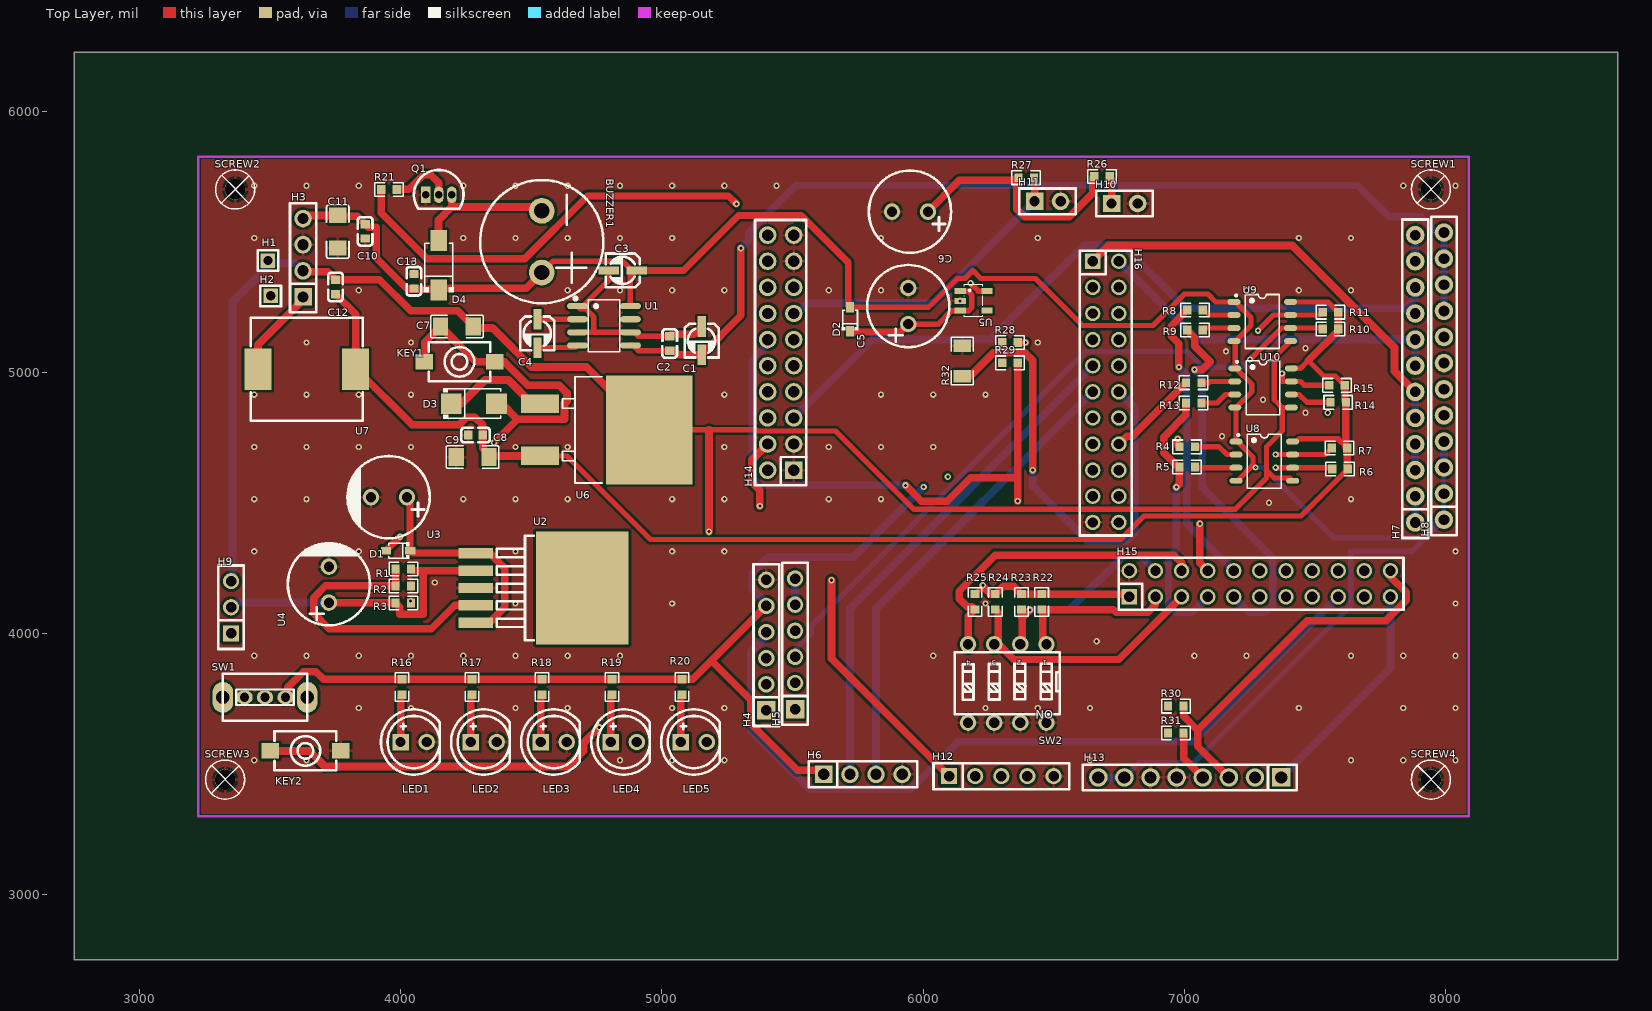
[diagram p0: Top Layer view]
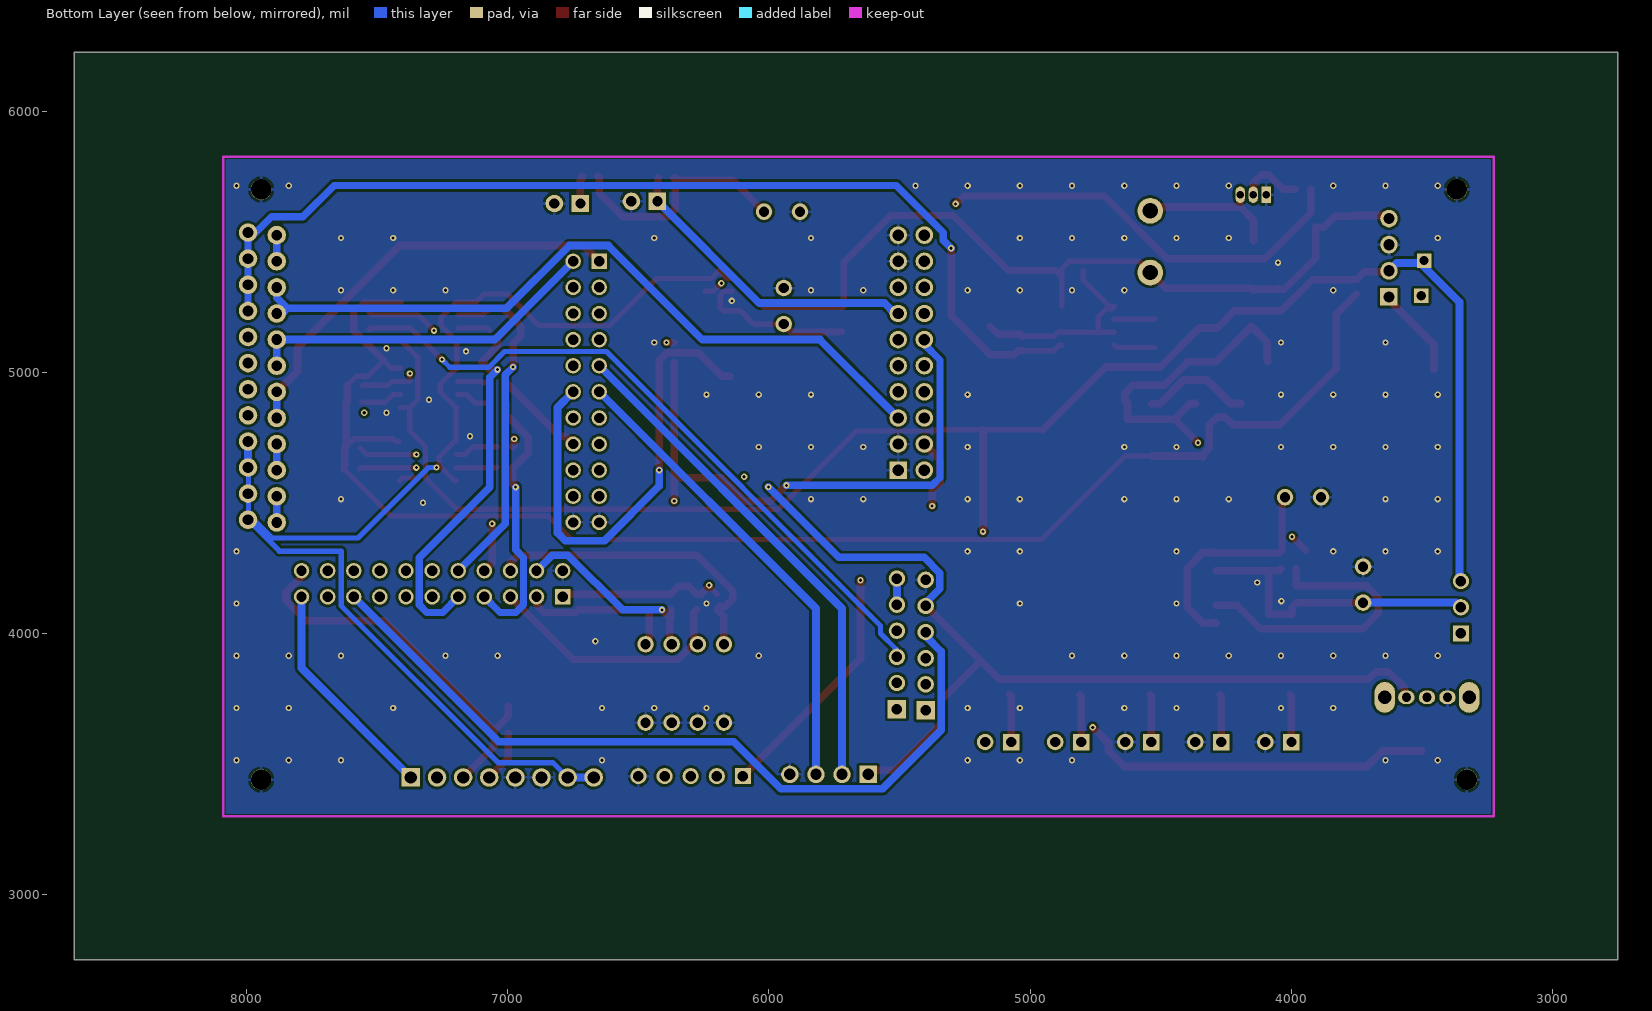
[diagram p1: Bottom Layer view, seen from below]
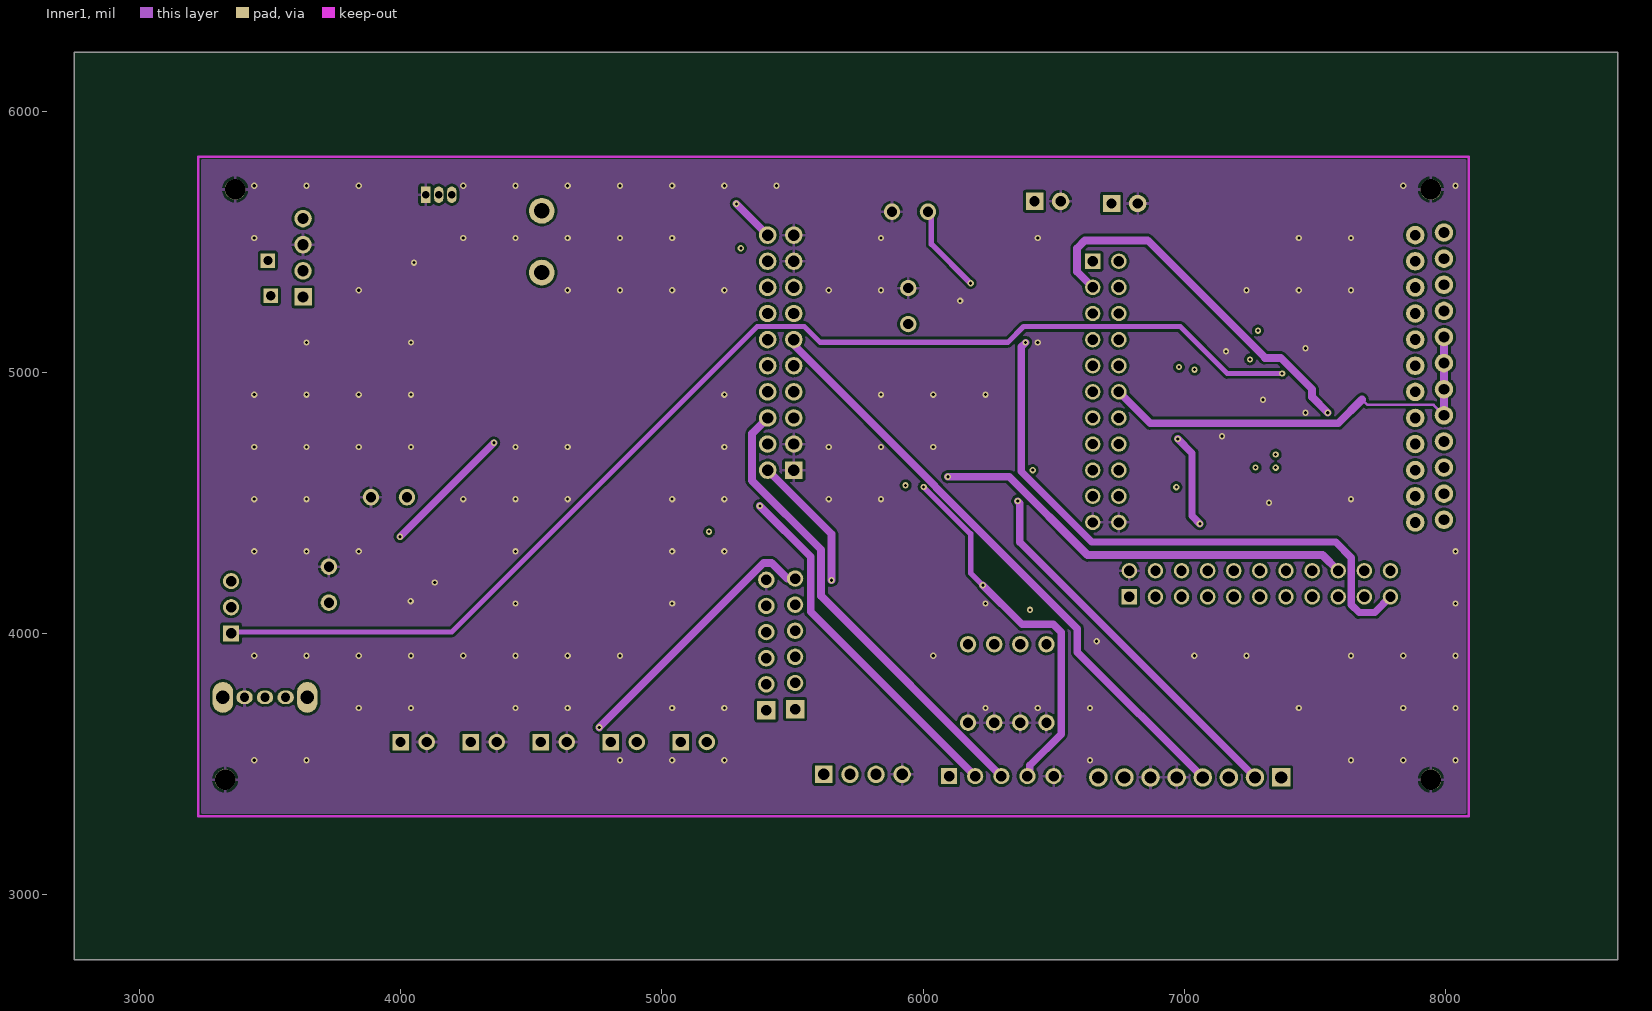
[diagram p2: Inner1]
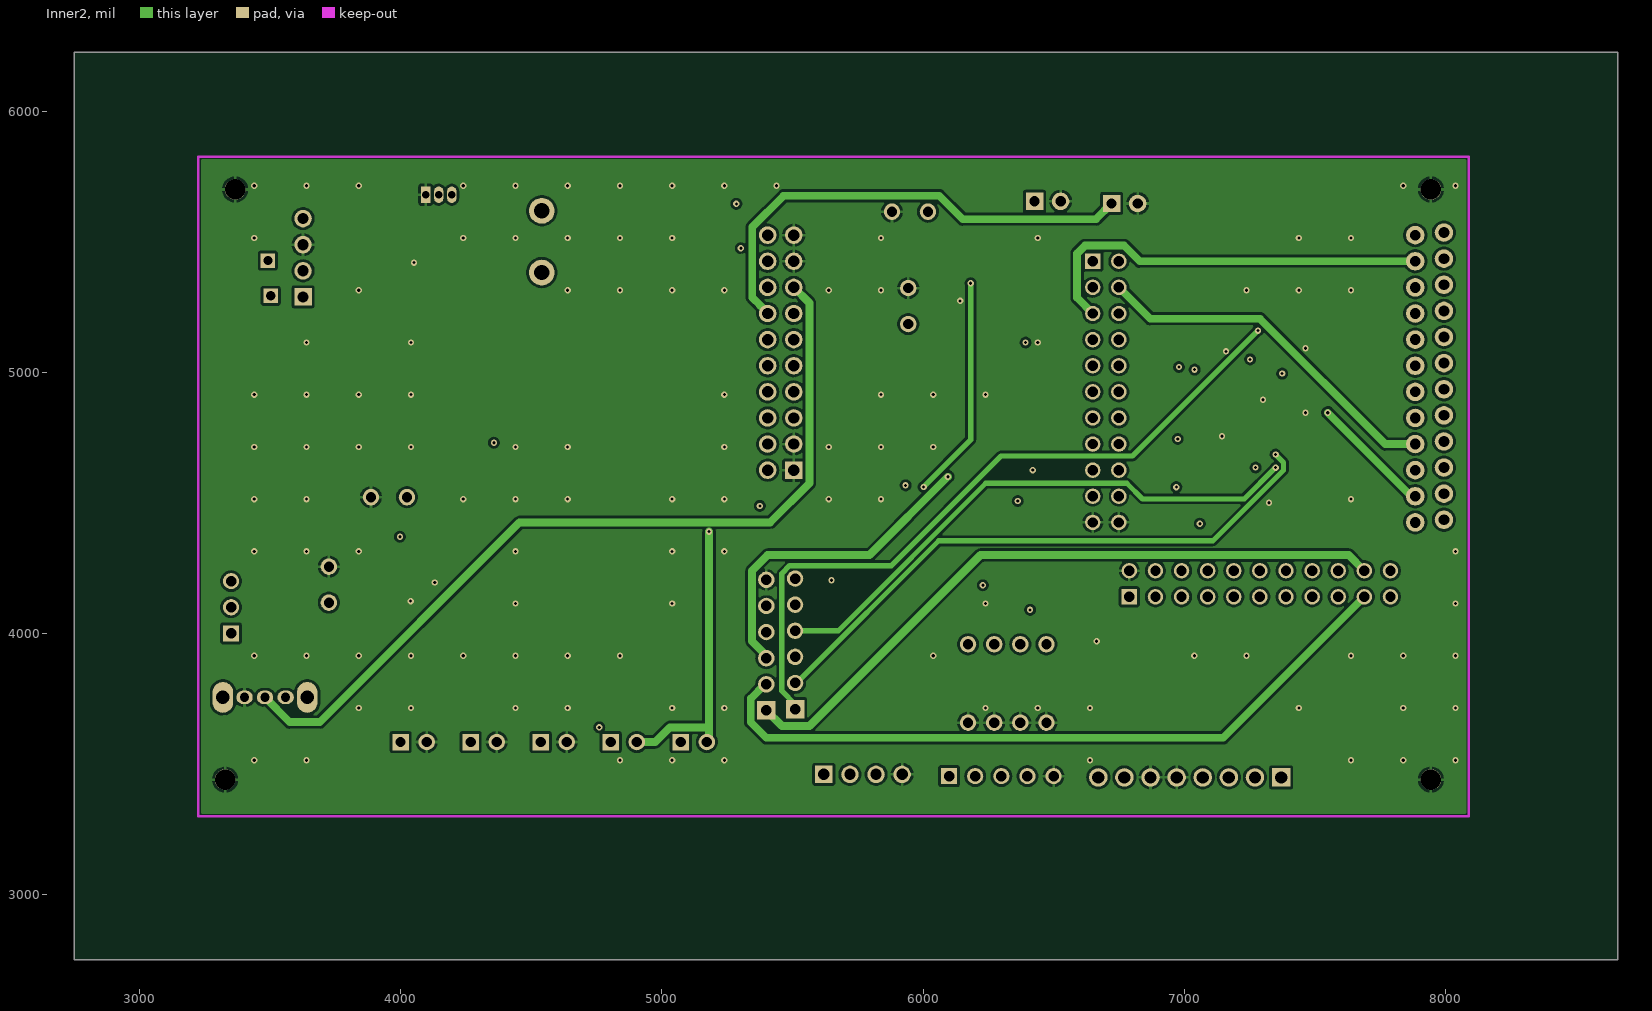
[diagram p3: Inner2]
# Altium PCB MISC75407.pcbdoc
Units mil, origin at the board's own origin, x right, y up, seen from the top; angles counter-clockwise.
Board outline 5910 x 3475 mil, 4 copper layers (Top Layer, Inner1, Inner2, Bottom Layer), stack 62.447 mil thick; 90 components, 74 nets, 316 pads, 149 vias.

## Layer stack, top to bottom
Top Layer: signal copper 1.378
Dielectric1: surface 8.283, 7628 RC49% 8.6mil, Dk 0
Inner1: signal copper 0.598
Dielectric2: surface 41.929, 1.1mm H/HOZ Copper, Dk 0
Inner2: signal copper 0.598
Dielectric3: surface 8.283, 7628 RC49% 8.6mil, Dk 0
Bottom Layer: signal copper 1.378

## Board outline
8660,2750 2750,2750 2750,6225 8660,6225

## Design rules (kind name [scope] priority, off if disabled: settings)
BoardOutlineClearance copperThickness2oz_1 [All] p2 off: genericclearance=7.99 ignorepadtopadclearanceinfootprint=FALSE except(0: Arc-SplitContinuation Track-SplitContinuation SMDPad-SplitContinuation THPad-SplitContinuation Via-SplitContinuation Fill-SplitContinuation Region-SplitContinuation Poly-SplitContinuation Text-SplitContinuation Hole-SplitContinuation; 5.98: Arc-CutoutEdge SMDPad-CutoutEdge THPad-CutoutEdge Via-CutoutEdge Fill-CutoutEdge Region-CutoutEdge Text-CutoutEdge; 6.93: Hole-OutlineEdge Hole-CutoutEdge; 10: Poly-OutlineEdge Poly-CutoutEdge; 11.81: Arc-OutlineEdge Track-OutlineEdge SMDPad-OutlineEdge THPad-OutlineEdge Via-OutlineEdge Fill-OutlineEdge Region-OutlineEdge Text-OutlineEdge Track-CutoutEdge)
BoardOutlineClearance copperThickness1oz_1 [All] p4: genericclearance=4.02 ignorepadtopadclearanceinfootprint=FALSE except(0: Arc-SplitContinuation Track-SplitContinuation SMDPad-SplitContinuation THPad-SplitContinuation Via-SplitContinuation Fill-SplitContinuation Region-SplitContinuation Poly-SplitContinuation Text-SplitContinuation Hole-SplitContinuation; 6: SMDPad-CutoutEdge THPad-CutoutEdge Via-CutoutEdge Fill-CutoutEdge Region-CutoutEdge Text-CutoutEdge; 6.93: Hole-OutlineEdge Hole-CutoutEdge; 10: Poly-OutlineEdge Poly-CutoutEdge; 11.8: Arc-OutlineEdge Track-OutlineEdge SMDPad-OutlineEdge THPad-OutlineEdge Via-OutlineEdge Fill-OutlineEdge Region-OutlineEdge Text-OutlineEdge; 11.81: Arc-CutoutEdge Track-CutoutEdge)
Clearance copperThickness2oz [All] p1 off: gap=7.99 ignorepadtopadclearanceinfootprint=FALSE except(5.98: SMDPad-Track SMDPad-SMDPad THPad-Track SMDPad-THPad THPad-THPad Track-Via SMDPad-Via THPad-Via Via-Via Fill-Track Region-Track Fill-SMDPad Region-SMDPad Fill-THPad Region-THPad Fill-Via Region-Via Fill-Fill Fill-Region Region-Region Arc-Track Arc-SMDPad Arc-THPad Arc-Via Fill-Arc Region-Arc Arc-Arc Text-Track SMDPad-Text Text-THPad Text-Via Fill-Text Region-Text Arc-Text Text-Text; 6.93: Hole-Track Hole-SMDPad Hole-THPad Hole-Via Fill-Hole Region-Hole Hole-Arc Hole-Text; 10: Poly-Track Poly-SMDPad Poly-THPad Poly-Via Poly-Fill Poly-Region Poly-Poly Poly-Arc Poly-Text Poly-Hole)
Clearance copperThickness1oz [All] p3: gap=4.02 ignorepadtopadclearanceinfootprint=FALSE except(5.98: SMDPad-Track SMDPad-SMDPad THPad-Track SMDPad-THPad THPad-THPad Track-Via SMDPad-Via THPad-Via Via-Via Fill-Track Region-Track Fill-SMDPad Region-SMDPad Fill-THPad Region-THPad Fill-Via Region-Via Fill-Fill Fill-Region Region-Region; 6: Arc-Track Arc-SMDPad Arc-THPad Arc-Via Fill-Arc Region-Arc Arc-Arc Text-Track SMDPad-Text Text-THPad Text-Via Fill-Text Region-Text Arc-Text Text-Text; 6.93: Hole-Track Hole-SMDPad Hole-THPad Hole-Via Fill-Hole Region-Hole Hole-Arc Hole-Text; 10: Poly-Track Poly-SMDPad Poly-THPad Poly-Via Poly-Fill Poly-Region Poly-Poly Poly-Arc Poly-Text Poly-Hole)
DiffPairsRouting differentialPair [All] p1: maxlimit=6 minlimit=6 mostfreqgap=6 toplayer_minwidth=5 toplayer_prefwidth=10 toplayer_maxwidth=100 toplayer_mingap=6 toplayer_prefgap=6 toplayer_maxgap=6 midlayer1_minwidth=5 midlayer1_prefwidth=10 midlayer1_maxwidth=100 midlayer1_mingap=6 midlayer1_prefgap=6 midlayer1_maxgap=6 midlayer2_minwidth=5 midlayer2_prefwidth=10 midlayer2_maxwidth=100 midlayer2_mingap=6 midlayer2_prefgap=6 midlayer2_maxgap=6 bottomlayer_minwidth=5 bottomlayer_prefwidth=10 bottomlayer_maxwidth=100 bottomlayer_mingap=6 bottomlayer_prefgap=6 bottomlayer_maxgap=6 maxuncoupledlength=10
HoleToHoleClearance otherClearance [All] p1: gap=11.81 allowstackedmicrovias=TRUE
Length netLength [All] p1: minlimit=0 maxlimit=0
MatchedLengths netLengthTolerance [All] p1: tolerance=1000
PasteMaskExpansion pasteMaskExpansion [All] p1: expansion=0
PlaneConnect innerPlane [All] p1: planeconnectstyle=Relief reliefexpansion=20 reliefentries=4 reliefconductorwidth=10 reliefairgap=10
PolygonConnect copperRegion [(InNet('GND'))] p1: connectstyle=Relief reliefconductorwidth=10 reliefentries=4 polygonreliefangle="90 Angle" airgapwidth=10 via.connectstyle=Relief via.reliefconductorwidth=10 via.reliefentries=4 via.polygonreliefangle="90 Angle" via.airgapwidth=10
RoutingVias viaSize [All] p1: holewidth=12.01 width=24.02 viastyle="Through Hole" minholewidth=11.81 minwidth=19.68 maxholewidth=248.03 maxwidth=393.7
SolderMaskExpansion solderMaskExpansion [IsVia] p1: expansion=-1000 istentingtop=TRUE
SolderMaskExpansion solderMaskExpansion [All] p2: expansion=2 istentingtop=FALSE
Width copperThickness2oz_2 [All] p1 off: maxlimit=100 minlimit=8 preferedwidth=10
Width copperThickness1oz_2 [All] p2: maxlimit=10 minlimit=10 preferedwidth=10 toplayer_minwidth=5 toplayer_maxwidth=100 toplayer_prefwidth=30 midlayer1_minwidth=5 midlayer1_maxwidth=100 midlayer1_prefwidth=30 midlayer2_minwidth=5 midlayer2_maxwidth=100 midlayer2_prefwidth=30 bottomlayer_minwidth=5 bottomlayer_maxwidth=100 bottomlayer_prefwidth=30

## Components (designator, comment, footprint, x,y, rotation, side; value= is the part's Value field where it differs from the comment)
BUZZER1 "buzzer" BUZ-TH_BD12.0-P6.00-D0.9-RD 4540,5500 r270 top
C1 "100uF" C_Ele_SMD_3x5.4mm 5151.69,5121.18 r90 top
C2 "100nF" C0603 5030,5110 r270 top
C3 "10uF" C_Ele_SMD_3x5.4mm 4849.45,5390.15 r0 top
C4 "47uF" C_Ele_SMD_3x5.4mm 4522.78,5148.38 r90 top
C5 "4.7uF" CAP-TH_BD8.0-P3.50-D0.5-FD_4.7UF400V8X14FS 5943.42,5253.46 r90 top
C6 "4.7uF" CAP-TH_BD8.0-P3.50-D0.5-FD_4.7UF400V8X14FS 5950,5615 r180 top
C7 "47UF" C1206 4215,5175 r0 top
C8 "100nF" C0603 4286.22,4759.27 r0 top
C9 "22UF" C1206 4275,4675 r0 top
C10 "100nF" C0603 3863.58,5539.45 r90 top
C11 "22UF" C1206 3758.58,5538.19 r90 top
C12 "4.7UF" C0603 3749.89,5326.65 r270 top
C13 "100nF" C0603 4050.19,5348.55 r270 top
D1 "1N5819WS" SOD-323_L1.8-W1.3-LS2.5-RD 3989.75,4316.72 r180 top
D2 "1N5819WS" SOD-323_L1.8-W1.3-LS2.5-RD 5720.39,5202.68 r90 top
D3 "SS34" SMA_L4.3-W2.6-LS5.2-RD 4280,4880 r0 top
D4 "SS34" SMA_L4.3-W2.6-LS5.0-RD 4145.32,5409.77 r90 top
H1 "" HDR-TH_1P-V-M_XKB_X4611WV-01I-C28D40 3491.11,5427.5 r90 top
H2 "" HDR-TH_1P-V-M_XKB_X4611WV-01I-C28D40 3501.86,5292.5 r90 top
H3 "" HDR-TH_4P-P2.54-V-F 3625.64,5438.48 r90 top
H4 "" HDR-TH_6P-P2.54-V-F 5400,3955 r90 top
H5 "" HDR-TH_6P-P2.54-V-F 5510,3960 r90 top
H6 "" HDR-TH_4P-P2.54-V-F 5770,3460 r0 top
H7 "" HDR-TH_12P-P2.54-V-F 7885,4975 r90 top
H8 "" HDR-TH_12P-P2.54-V-F 7995,4985 r90 top
H9 "" HDR-TH_3P-P2.54-V-F 3350,4100 r90 top
H10 "" HDR-TH_2P-P2.54-V-F 6771.95,5646.21 r0 top
H11 "" HDR-TH_2P-P2.54-V-F 6476.95,5654.61 r0 top
H12 "" HDR-TH_5P-P2.54-V-F 6299.85,3453.3 r0 top
H13 "" HDR-TH_8P-P2.54-V-F-1 7021.22,3448.3 r180 top
H14 "" HDR-TH_20P-P2.54-V-R2-C10-S2.54 5455,5075 r90 top
H15 "CS-1106-2*11B" HDR-TH_22P-P2.54-V-M-R2-C11-S2.54-1 7290,4190 r0 top
H16 "CS-1106-2*11B" HDR-TH_22P-P2.54-V-M-R2-C11-S2.54-1 6700,4925 r270 top
KEY1 "SW-SPST" KEY-SMD_L6.0-W3.6-LS8.0 4225,5040 r0 top
KEY2 "SW-SPST" KEY-SMD_L6.0-W3.6-LS8.0 3635,3550 r0 top
LED1 "" LED-TH_5mm 4049.26,3583.93 r0 top
LED2 "" LED-TH_5mm 4317.5,3583.93 r0 top
LED3 "" LED-TH_5mm 4585.73,3583.93 r0 top
LED4 "" LED-TH_5mm 4853.97,3583.93 r0 top
LED5 "" LED-TH_5mm 5122.21,3583.93 r0 top
Q1 "" S8050_TO_92 4145.32,5679.77 r0 top
R1 "3.9K" R0603 4009.75,4246.72 r0 top
R2 "1K" R0603 4009.75,4181.72 r180 top
R3 "1K" R0603 4009.75,4116.72 r180 top
R4 "1K" R0603 7011.46,4714.67 r180 top
R5 "1K" R0603 7011.46,4636.97 r180 top
R6 "1K" R0603 7597.22,4629.26 r0 top
R7 "1K" R0603 7595,4710 r0 top
R8 "1K" R0603 7041.46,5238.93 r180 top
R9 "1K" R0603 7041.46,5161.22 r180 top
R10 "1K" R0603 7560,5165 r0 top
R11 "1K" R0603 7560,5230 r0 top
R12 "1K" R0603 7036.46,4959.87 r180 top
R13 "1K" R0603 7036.46,4882.17 r180 top
R14 "1K" R0603 7590,4885 r0 top
R15 "1K" R0603 7585,4950 r0 top
R16 "1K" R0603 4004.26,3794.27 r90 top
R17 "1K" R0603 4272.5,3794.27 r90 top
R18 "1K" R0603 4540.73,3794.27 r90 top
R19 "3.3K" R0603 4808.97,3794.27 r90 top
R20 "3.3K" R0603 5077.21,3794.27 r90 top
R21 "1K" R0603 3955,5700 r0 top
R22 "1K" R0603 6454.43,4120.95 r270 top
R23 "1K" R0603 6376.73,4120.95 r270 top
R24 "1K" R0603 6276.73,4120.95 r270 top
R25 "1K" R0603 6199.03,4120.95 r270 top
R26 "1K" R0603 6685,5750 r0 top
R27 "1K" R0603 6395,5745 r0 top
R28 "1K" R0603 6333.02,5113.91 r0 top
R29 "1K" R0603 6333.02,5036.21 r0 top
R30 "1K" R0603 6968.02,3721.21 r0 top
R31 "1K" R0603 6968.02,3618.3 r0 top
R32 "100mΩ" R1206 6150.34,5042.73 r90 top
SCREW1 "" M2螺丝 7945,5700 r0 top
SCREW2 "" M2螺丝 3365.64,5700 r0 top
SCREW3 "" M2螺丝 3327.21,3440 r0 top
SCREW4 "" M2螺丝 7945,3440 r0 top
SW1 "" 拨动开关 3475,3755 r0 top
SW2 "DIP switch EI-04" SW-TH_DIPSWITCHEI-04 6322.49,3808.25 r180 top
U1 "LM2663M" SOIC-8_L4.9-W3.9-P1.27-LS6.0-BL 4778.16,5178.03 r270 top
U2 "MIC29302" TO-263-5_L10.1-W8.7-P1.70-LS15.2-BR 4491.27,4173.77 r180 top
U3 "22UF400V" CAP-TH_BD8.0-P3.50-D0.6-FD 3954.75,4521.72 r180 top
U4 "22UF400V" CAP-TH_BD8.0-P3.50-D0.6-FD 3724.75,4186.72 r90 top
U5 "TPS73633DBVR" SOT-23-5_L3.0-W1.7-P0.95-LS2.8-BR 6193.42,5273.46 r180 top
U6 "LM2940HR-5.0" TO-263-2_L10.1-W9.1-P5.08-LS15.2-BR 4742.21,4779.67 r180 top
U7 "6.8UH" IND-SMD_L10.9-W10.0_ACL1009 3639.89,5011.65 r180 top
U8 "HCPL-0631-000E" SO-8_L5.1-W3.9-P1.27-LS6.0-BL 7307.06,4659.67 r270 top
U9 "HCPL-0631-000E" SO-8_L5.1-W3.9-P1.27-LS6.0-BL 7299.26,5194.26 r270 top
U10 "HCPL-0631-000E" SO-8_L5.1-W3.9-P1.27-LS6.0-BL 7302.06,4939.87 r270 top

## Footprints (in the part's own frame and the unit in brackets; to place one, negate y for a bottom-side part, rotate by r counter-clockwise, add the part's x,y. Pads: shape width x height; smd on the part's side, far side on the other; paste and mask are expansions set on the pad)
BUZ-TH_BD12.0-P6.00-D0.9-RD [mm]
  round 2.5 hole 1.5 paste+0 mask+0.05: 1(-3,0) 2(3,0)
  silkscreen extent -5.99,-5.99 5.99,5.99
C0603 [mm]
  rect 0.8x0.9 smd: 1(-0.7,0) 2(0.7,0)
  silkscreen extent -1.39,-0.71 1.39,0.71
C1206 [mm]
  rect 1.485x1.728 smd paste-100 mask+0.051: 1(-1.593,0) 2(1.593,0)
  silkscreen extent -2.56,-1.09 2.56,1.09
C_Ele_SMD_3x5.4mm [mil]
  rect 78.7x31.5 smd paste+0 mask+2: 1(54.1,-0.55) 2(-53.7,-0.55)
  silkscreen extent -65,-65 65,65
CAP-TH_BD8.0-P3.50-D0.5-FD_4.7UF400V8X14FS [mm]
  round 1.6 hole 1: 1(-1.75,0) 2(1.75,0)
  silkscreen extent -4,-4 4,4
CAP-TH_BD8.0-P3.50-D0.6-FD [mm]
  round 1.6 hole 1: 1(-1.75,0) 2(1.75,0)
  silkscreen extent -3.96,-4 4.04,4
HDR-TH_1P-V-M_XKB_X4611WV-01I-C28D40 [mm]
  rect 1.4x1.4 hole 0.9: 1(0,0)
  silkscreen extent -1,-1 1,1
HDR-TH_2P-P2.54-V-F [mm]
  rect 1.7x1.7 hole 1: 1(-1.27,0)
  round 1.7 hole 1: 2(1.27,0)
  silkscreen extent -2.74,-1.25 2.74,1.25
HDR-TH_3P-P2.54-V-F [mil]
  rect 62x62 hole 40.16: 1(-100,0)
  round 62 hole 40.16: 2(0,0) 3(100,0)
  silkscreen extent -160,-49 160,49
HDR-TH_4P-P2.54-V-F [mm]
  rect 1.7x1.7 hole 1.1: 1(-3.81,0)
  round 1.7 hole 1.1: 2(-1.27,0) 3(1.27,0) 4(3.81,0)
  silkscreen extent -5.29,-1.27 5.29,1.27
HDR-TH_5P-P2.54-V-F [mil]
  rect 62x62 hole 40.16: 1(-200,0)
  round 62 hole 40.16: 2(-100,0) 3(0,0) 4(100,0) 5(200,0)
  silkscreen extent -260,-50 260,50
HDR-TH_6P-P2.54-V-F [mm]
  rect 1.8x1.8 hole 1.02: 1(-6.35,0)
  round 1.6 hole 1.02: 2(-3.81,0) 3(-1.27,0) 4(1.27,0) 5(3.81,0) 6(6.35,0)
  silkscreen extent -7.87,-1.25 7.87,1.25
HDR-TH_8P-P2.54-V-F-1 [mm]
  rect 1.8x1.8 hole 1.2: 1(-8.89,0)
  round 1.8 hole 1.2: 2(-6.35,0) 3(-3.81,0) 4(-1.27,0) 5(1.27,0) 6(3.81,0) 7(6.35,0) 8(8.89,0)
  silkscreen extent -10.41,-1.25 10.41,1.25
HDR-TH_12P-P2.54-V-F [mm]
  round 1.8 hole 1.05: 1(-13.97,0) 2(-11.43,0) 3(-8.89,0) 4(-6.35,0) 5(-3.81,0) 6(-1.27,0) 7(1.27,0) 8(3.81,0) 9(6.35,0) 10(8.89,0) 11(11.43,0) 12(13.97,0)
  silkscreen extent -15.49,-1.25 15.49,1.25
HDR-TH_20P-P2.54-V-R2-C10-S2.54 [mm]
  rect 1.7x1.7 hole 1.1: 1(-11.43,-1.27)
  round 1.7 hole 1.1: 2(-11.43,1.27) 3(-8.89,-1.27) 4(-8.89,1.27) 5(-6.35,-1.27) 6(-6.35,1.27) 7(-3.81,-1.27) 8(-3.81,1.27) 9(-1.27,-1.27) 10(-1.27,1.27) 11(1.27,-1.27) 12(1.27,1.27) 13(3.81,-1.27) 14(3.81,1.27) 15(6.35,-1.27) 16(6.35,1.27) 17(8.89,-1.27) 18(8.89,1.27) 19(11.43,-1.27) 20(11.43,1.27)
  silkscreen extent -12.9,-2.54 12.9,2.5
HDR-TH_22P-P2.54-V-M-R2-C11-S2.54-1 [mm]
  rect 1.5x1.5 hole 1: 1(-12.7,-1.27)
  round 1.5 hole 1: 2(-12.7,1.27) 3(-10.16,-1.27) 4(-10.16,1.27) 5(-7.62,-1.27) 6(-7.62,1.27) 7(-5.08,-1.27) 8(-5.08,1.27) 9(-2.54,-1.27) 10(-2.54,1.27) 11(0,-1.27) 12(0,1.27) 13(2.54,-1.27) 14(2.54,1.27) 15(5.08,-1.27) 16(5.08,1.27) 17(7.62,-1.27) 18(7.62,1.27) 19(10.16,-1.27) 20(10.16,1.27) 21(12.7,-1.27) 22(12.7,1.27)
  silkscreen extent -13.72,-2.54 13.97,2.54
IND-SMD_L10.9-W10.0_ACL1009 [mm]
  rect 2.6x4 smd: 1(-4.75,0) 2(4.75,0)
  silkscreen extent -5.45,-5 5.45,5
KEY-SMD_L6.0-W3.6-LS8.0 [mm]
  rect 1.7x1.5 smd: 1(-3.431,0) 2(3.431,0)
  silkscreen extent -3.01,-1.9 2.99,1.9
LED-TH_5mm [mm]
  rect 1.6x1.6 hole 1 paste+0 mask+0.051: 1(-1.27,0)
  round 1.6 hole 1 paste+0 mask+0.051: 2(1.27,0)
  silkscreen extent -3.17,-3.17 2.54,3.17
M2螺丝 [mm]
  round 2 hole 2: 1(0,0)
  silkscreen extent -1.9,-1.9 1.9,1.9
R0603 [mil]
  rect 31.75x34.02 smd paste-3937.01 mask+2: 1(-29.66,0) 2(29.66,0)
  silkscreen extent -55,-26 55,26
R1206 [mil]
  rect 47.54x66.97 smd paste-3937.01 mask+2: 1(-58.22,0) 2(58.22,0)
  silkscreen extent -91,-42 91,42
S8050_TO_92 [mil]
  rect 35.4x63 hole 27.6 paste+0 mask+2: 1(-50,0)
  oval 35.4x63 hole 27.6 paste+0 mask+2: 2(0,0) 3(50,0)
  silkscreen extent -95,-53 95,95
SMA_L4.3-W2.6-LS5.0-RD [mm]
  rect 2.046x1.62 smd: 1(-2.404,-0.009) 2(2.404,0.009)
  silkscreen extent -2.61,-1.44 2.16,1.44
SMA_L4.3-W2.6-LS5.2-RD [mm]
  rect 2x2 smd: 1(-2.2,0) 2(2.2,0)
  silkscreen extent -2.98,-1.5 2.6,1.5
SO-8_L5.1-W3.9-P1.27-LS6.0-BL [mil]
  oval 22.38x50 smd: 1(-75,-108.27) 2(-25,-108.27) 3(25,-108.27) 4(75,-108.27) 5(75,108.27) 6(25,108.27) 7(-25,108.27) 8(-75,108.27)
  silkscreen extent -104,-104 103,65
SOD-323_L1.8-W1.3-LS2.5-RD [mm]
  rect 1x0.75 smd: 1(-1.173,0) 2(1.173,0)
  silkscreen extent -1.08,-0.8 0.9,0.8
SOIC-8_L4.9-W3.9-P1.27-LS6.0-BL [mm]
  oval 0.588x2.045 smd: 1(-1.905,-2.57) 2(-0.635,-2.57) 3(0.635,-2.57) 4(1.905,-2.57) 5(1.905,2.57) 6(0.635,2.57) 7(-0.635,2.57) 8(-1.905,2.57)
  silkscreen extent -2.8,-2.92 2.53,1.52
SOT-23-5_L3.0-W1.7-P0.95-LS2.8-BR [mm]
  rect 1.1x0.6 smd: 1(1.3,-0.95) 2(1.3,0) 3(1.3,0.95) 4(-1.3,0.95) 5(-1.3,-0.95)
  silkscreen extent -0.9,-1.55 0.9,1.55
SW-TH_DIPSWITCHEI-04 [mm]
  round 1.6 hole 1: 1(-3.81,-3.81) 2(-1.27,-3.81) 3(1.27,-3.81) 4(3.81,-3.81) 5(3.81,3.81) 6(1.27,3.81) 7(-1.27,3.81) 8(-3.81,3.81)
  silkscreen extent -5.1,-3.05 5.11,2.98
TO-263-2_L10.1-W9.1-P5.08-LS15.2-BR [mm]
  rect 3.7x1.8 smd: 1(5.321,-2.54) 3(5.321,2.54)
  rect 8.4x10.608 smd: 2(-5.321,0)
  silkscreen extent -0.75,-5.18 3.12,5.18
TO-263-5_L10.1-W8.7-P1.70-LS15.2-BR [mm]
  rect 3.359x1.02 smd: 1(5.183,-3.4) 2(5.183,-1.7) 3(5.183,0) 4(5.183,1.7) 5(5.183,3.4)
  rect 9x11 smd: 6(-5.183,0)
  silkscreen extent -0.45,-5.1 3.15,5.1
拨动开关 [mil]
  oval 63x51.2 hole 35.4 paste+0 mask+2: 1(-73.4,0) 2(5,0) 3(84,0)
  oval 78.7x118.1 hole 51.2 paste+0 mask+2: 4(166.7,0) 5(-156.1,0)
  silkscreen extent -156,-90 167,90

## Via types
v1: diameter 24.02, hole 12, Top Layer to Bottom Layer, 149 vias

## Nets (pads, with @x,y where several pads share a name; then routed paths per layer and width w, separated by ;. In a path a pad name is that pad's centre, name@x,y a point inside that pad or via, vN(x,y) a via of type N, cw(c..) or ccw(c..) an arc to the next point about the centre after c; other vN are vias at no path point)
$1N2: C1.1 C2.1 C3.2 U1.1 U1.3 U1.6 | length 833.4
  Top Layer w20.84: U1.3 U1.6 4894.53,5153.03 4910,5137.56 C2.1 ; 4738.67,5153.03 4738.67,5213.03 4708.67,5243.03 4686.98,5243.03 U1.1 4697.66,5253.03 4795.75,5351.13 C3.2@4795.75,5389.6
  Top Layer w28.35: C2.1 5037.73,5145.28 5122.24,5145.28 C1.1
$1N4: C4.1 U1.2 | length 153.7
  Top Layer w20.84: C4.1 4673.34,5202.48 U1.2
$1N5: C4.2 U1.4 | length 157.1
  Top Layer w20.84: C4.2 4668.63,5094.68 U1.4
$1N6: D1.1 U2.1 U2.5 U3.1 | length 888
  Top Layer w26.58: U3.1 4023.65,4508.99 4035.91,4496.72 D1.1 4045,4307.63 U2.1
  Top Layer w30: U2.5 4338.32,4039.91 4398.32,4099.91 4398.32,4249.91 4338.32,4309.91 4289.49,4309.91 U2.1
$1N10: R1.1 R2.2 U2.4 | length 1139.4
  Top Layer w28.58: R1.1 R2.2 3711.69,4181.72 3666.81,4136.84 3666.81,4076.84 3726.81,4016.84 4116.81,4016.84 4206.81,4106.84 U2.4
$1N12: C5.1 D2.1 U5.1 U5.3 | length 604.2
  Top Layer w21.26: C5.1 6058.46,5184.56 6109.96,5236.06 U5.3 6174.52,5236.06 6187.04,5248.58 6187.04,5296.06 6172.24,5310.86 U5.1
  Top Layer w26.58: D2.1 5733.43,5154.56 5913.42,5154.56 C5.1
$1N19: D3.1 U6.1 | length 414
  Top Layer w30: D3.1 4232.4,4880 4322.4,4970 4412.4,4970 4502.73,4879.67 U6.1
$1N27: H3.1 U7.2 | length 348.4
  Top Layer w30: U7.2 3452.89,5105.39 3625.64,5278.14 H3.1
$1N34: R4.1 U8.2 | length 170.1
  Top Layer w20.14: R4.1 7133.72,4714.67 7163.72,4684.67 U8.2
$1N35: R5.1 U8.3 | length 158.5
  Top Layer w20.14: R5.1 7043.72,4634.67 U8.3
$1N48: R9.1 U9.3 | length 123.2
  Top Layer w20.14: R9.1 7079.15,5169.26 U9.3
$1N49: R8.1 U9.2 | length 128
  Top Layer w20.14: R8.1 7076.25,5238.93 7095.92,5219.26 U9.2
$1N54: R14.1 U10.6 | length 162.4
  Top Layer w20.14: U10.6 7440.33,4914.87 7470.33,4884.87 R14.1
$1N58: R13.1 U10.3 | length 141.2
  Top Layer w20.14: R13.1 7126.02,4882.17 7158.72,4914.87 U10.3
$1N59: R12.1 U10.2 | length 129.7
  Top Layer w20.14: R12.1 7093.72,4959.87 7098.72,4964.87 U10.2
$1N62: LED1.1 R16.1 | length 182.7
  Top Layer w28.58: LED1.1 3999.26,3759.6 R16.1
$1N65: LED2.1 R17.1 | length 182.7
  Top Layer w28.58: LED2.1 4267.5,3759.6 R17.1
$1N67: LED3.1 R18.1 | length 182.7
  Top Layer w28.58: LED3.1 4535.73,3759.6 R18.1
$1N70: LED4.1 R19.1 | length 182.7
  Top Layer w28.58: LED4.1 4803.97,3759.6 R19.1
$1N73: LED5.1 R20.1 | length 182.7
  Top Layer w28.58: LED5.1 5072.21,3759.6 R20.1
$1N74: BUZZER1.1 D4.2 Q1.3 | length 547.4
  Top Layer w30: D4.2 4144.95,5583 4195.32,5633.37 ; Q1.3 4195.32,5633.37 ; BUZZER1.1 4525.32,5633.37 4195.32,5633.37
$1N76: Q1.2 R21.2 | length 241.7
  Top Layer w28.58: R21.2 4029.86,5700 4085.32,5755.46 4115.32,5755.46 4145.32,5725.46 Q1.2
$1N100: H5.5 H5.6 KEY2.1 | length 2500.4
  Top Layer w30: KEY2.1 3650,3550 3710,3490 4640,3490 4700,3550 4700,3580 v1(4760,3640)
  Inner1 w30: v1(4760,3640) 5390,4270 5420,4270 5480,4210 H5.6
  Bottom Layer w30: H5.5 H5.6
A1: H16.7
ADB2: H7.9 H7.10 H14.5 | length 2857.6
  Bottom Layer w30: H14.5 5805,5125 6255,5125 6615,5485 6765,5485 7005,5245 7845,5245 ; H7.9 7865,5225 7845,5245 ; H7.10 7885,5285 7845,5245
ADE20: H7.1 H7.2 H16.3 | length 2005.8
  Inner1 w30: H16.3 6590,5385 6590,5475 6620,5505 6860,5505 7310,5055 7370,5055 7490,4935 7490,4905 v1(7550,4845)
  Inner2 w30: v1(7550,4845) 7870,4525 H7.2
  Bottom Layer w30: H7.1 H7.2
ADE21: H7.3 H7.4 H16.4 | length 1483.5
  Inner2 w30: H16.4 6870,5205 7290,5205 7770,4725 H7.4
  Bottom Layer w30: H7.3 H7.4
ADE22: H7.5 H7.6 H16.1 | length 1644.5
  Top Layer w30: H16.1 6710,5485 7415,5485 7805,5095 7805,5005 H7.6
  Bottom Layer w30: H7.5 H7.6
ADE23: H7.7 H7.8 H16.2 | length 1359.3
  Bottom Layer w30: H16.2 7050,5125 H7.8 H7.7
ADE29: H16.6
ADE30: H7.11 H7.12 H16.5 | length 1687.1
  Inner2 w30: H16.5 6590,5285 6590,5455 6620,5485 6770,5485 6830,5425 H7.11
  Bottom Layer w30: H7.11 H7.12
AGND: H8.5 H8.6 H8.7 H8.8 H16.12 R32.1 | length 3511.2
  Top Layer w30: R32.1 6180,4985 6270,5075 6390,5075 6420,5045 v1(6420,4625)
  Inner1 w10: 7680.87,4895.87 7701.74,4875 7955,4875 H8.5
  Inner1 w30: H16.12 6870,4805 7590,4805 7680.87,4895.87 ; H8.5 H8.6 H8.7 H8.8
  Bottom Layer w30: v1(6420,4625) 6420,4565 6630,4355 6780,4355 6810,4385 6810,4865 H16.12
B16: H13.4 H14.11 R31.2 | length 2525.9
  Top Layer w28.58: R31.2 6997.69,3521.84 H13.4
  Inner1 w28.58: H14.11 5505,5104.52 6591.22,4018.3 6591.22,3928.3 H13.4
B17: H13.2 H14.12 R29.2 | length 3609.5
  Top Layer w28.58: v1(5933.16,4566.84) 5993.16,4506.84 6092.68,4506.84 6182.68,4596.84 6362.68,4596.84 ; v1(6362.68,4506.84) 6362.68,4776.84 R29.2
  Inner1 w28.58: v1(6362.68,4506.84) 6371.22,4498.3 6371.22,4348.3 H13.2
  Bottom Layer w28.58: H14.12 5405,5106.84 5345,5046.84 5345,4596.84 5375,4566.84 v1(5933.16,4566.84)
C0: H14.15 SW1.2 | length 3278.2
  Inner2 w30: SW1.2 3575,3660 3690,3660 4455,4425 5415,4425 5565,4575 5565,5265 H14.15
C1: H14.16
C2: H14.18
C3: H14.20 R21.1 | length 1803.7
  Top Layer w28.58: R21.1 3925.34,5610 4100.34,5435 4475,5435 4715,5675 5255,5675 v1(5285,5645)
  Inner1 w28.58: v1(5285,5645) H14.20
C4: H13.3 H15.22 R30.2 | length 1487.9
  Top Layer w28.58: R30.2 6997.69,3681.84 7051.22,3628.3 ; H13.3 7051.22,3568.3 7051.22,3628.3 ; H15.22 7790,4217.09 7850,4157.09 7850,4127.09 7771.22,4048.3 7471.22,4048.3 7051.22,3628.3
C5: H13.1 H15.21 R28.2 | length 3163.1
  Top Layer w28.58: R28.2 v1(6392.68,5113.91)
  Inner1 w28.58: v1(6392.68,5113.91) 6376.6,5097.82 6376.6,4620 6646.6,4350 7580,4350 7640,4290 7640,4110 7670,4080 7730,4080 H15.21
  Bottom Layer w30: H13.1 7790,3867.09 H15.21
C6: H4.1 H15.20 | length 2611
  Inner2 w30: H4.1 5460,3645 5565,3645 6220,4300 7630,4300 H15.20
C7: H4.2 H15.19 | length 2771.3
  Inner2 w30: H4.2 5395,3805 5340,3750 5340,3660 5400,3600 7150,3600 H15.19
C8: H4.3 H15.18 | length 2901
  Inner1 w30: v1(6095,4600) 6330,4600 6630,4300 7530,4300 H15.18
  Inner2 w30: H4.3 5400,3915 5345,3970 5345,4240 5405,4300 5795,4300 v1(6095,4600)
C9: H4.4 H15.17 | length 3047.5
  Bottom Layer w30: H4.4 5400,3990 5340,3930 5340,3630.01 5565,3405 5955,3405 6135,3585 7035,3585 H15.17
CCDB0: H12.1 H14.2 | length 1459.5
  Top Layer w30: v1(5649.85,4203.3) 5649.85,3903.3 H12.1@6099.85,3453.3
  Inner1 w30: H14.2 5649.85,4380.15 v1(5649.85,4203.3)
CCDB1: H12.2 H14.4 | length 1650.6
  Top Layer w30: v1(5375,4488.15) 5375,4548.15 5345,4578.15 5345,4665 H14.4
  Inner1 w30: v1(5375,4488.15) 5569.85,4293.3 5569.85,4083.3 H12.2@6199.85,3453.3
CCDB3: H12.3 H14.6 | length 1792.1
  Inner1 w30: H14.6 5345,4765 5345,4585 5609.85,4320.15 5609.85,4143.3 H12.3@6299.85,3453.3
D4: H15.6 R25.2 SW2.4 | length 1201.5
  Top Layer w28.58: SW2.4 6172.49,4064.74 R25.2 6188.05,4102.26 6169.03,4102.26 6139.03,4132.26 6139.03,4162.26 6276.77,4300 6960,4300 6990,4270 H15.6
D5: H15.5 R24.2 SW2.3 | length 978.5
  Top Layer w28.58: SW2.3 6274.24,3960 SW2.3@6288.01,3960 ; R24.2 6288.01,4080 SW2.3@6288.01,3960 ; H15.5 6750,3900 6348.01,3900 SW2.3@6288.01,3960
D6: H15.4 R23.2 SW2.2 | length 770.9
  Top Layer w28.58: SW2.2 6380,3970 6380,4060 ; R23.2 6376.73,4063.27 6380,4060 ; v1(6410,4090) 6380,4060
  Bottom Layer w28.58: v1(6410,4090) 6560,4090 6770,4300 6830,4300 H15.4
D7: H15.3 R22.2 SW2.1 | length 621.6
  Top Layer w28.58: R22.2 6728.72,4091.28 6740,4080 6860,4080 6890,4110 H15.3 ; R22.2@6458.72,4091.28 6458.72,3971.28 SW2.1
GGND: C7.2 C12.1 H1.1 H3.2 H9.3 LED4.2 LED5.2 U6.2 U8.5 U9.5 U10.5 | length 7789.8
  Top Layer w20.14: U6.2 5360.47,4779.67 5365.27,4774.87 5665.26,4774.87 5965.26,4474.87 7195.26,4474.87 7315.26,4594.87 7315.26,4624.87 ; U9.5 7345.26,5056.99 7345.26,4894.87 7375.26,4864.87 ; U10.5 7375.26,4864.87 ; U8.5 7405.26,4594.87 7345.26,4594.87 7315.26,4624.87 ; 7315.26,4624.87 7315.26,4714.87 7375.26,4774.87 7375.26,4864.87
  Top Layer w28.35: H3.2 3629.89,5384.21 3719.89,5384.21 C12.1 3767.7,5355 3917.7,5355 4037.7,5235 4217.7,5235 C7.2
  Top Layer w30: C7.2 4283.03,5169.67 4351.68,5169.67 4501.68,5019.67 4711.68,5019.67 U6.2 ; v1(5180.47,4389.67) 5180.47,4779.67
  Inner2 w30: LED4.2 4974.73,3583.93 5030.47,3639.67 5180.47,3639.67 ; LED5.2 5180.47,3592.19 v1(5180.47,4389.67)
  Bottom Layer w30: H9.3 3355.64,4205.64 3355.64,5268.48 H1.1@3505.64,5418.48 ; H1.1 3496.61,5427.5 H1.1@3505.64,5418.48 ; H3.2 3595.64,5418.48 H1.1@3505.64,5418.48
GHGL: H11.1 H14.13 R27.2 | length 1190.4
  Top Layer w28.58: R27.2 6426.95,5714.61 H11.1
  Bottom Layer w30: H14.13 5517.33,5225 5556.95,5264.61 6036.95,5264.61 H11.1
GHGR: H10.1 H14.14 R26.2 | length 1949.3
  Top Layer w28.58: R26.2 6714.66,5743.49 6721.95,5736.21 H10.1
  Inner2 w30: H14.14 5376.21,5256.21 5346.21,5286.21 5346.21,5556.21 5466.21,5676.21 6061.95,5676.21 6151.95,5586.21 6661.95,5586.21 H10.1
GND: C5.2 C6.2 C8.1 C9.1 C10.1 C11.1 C13.1 H3.3 H4.6 H6.4 H10.2 H11.2 H12.5 H13.5 H13.6 H14.1 H14.3 H14.17 H14.19 H15.2 H16.21 H16.22 KEY2.2 LED1.2 LED2.2 LED3.2 Q1.1 R2.1 R3.1 R32.2 SCREW1.1 SCREW2.1 SCREW3.1 SCREW4.1 SW1.1 SW2.5 SW2.6 SW2.7 SW2.8 U2.3 U3.2 U4.2 U5.2
  other v1: 3439.1,3514.1 3639.1,3514.1 4839.1,3514.1 5039.1,3514.1 5239.1,3514.1 6639.1,3514.1 7639.1,3514.1 7839.1,3514.1 8039.1,3514.1 3839.1,3714.1 4039.1,3714.1 4439.1,3714.1 4639.1,3714.1 5039.1,3714.1 5239.1,3714.1 6239.1,3714.1 6439.1,3714.1 6639.1,3714.1 7439.1,3714.1 7839.1,3714.1 8039.1,3714.1 3439.1,3914.1 3639.1,3914.1 3839.1,3914.1 4039.1,3914.1 4239.1,3914.1 4439.1,3914.1 4639.1,3914.1 4839.1,3914.1 6039.1,3914.1 7039.1,3914.1 7239.1,3914.1 7639.1,3914.1 7839.1,3914.1 8039.1,3914.1 6665,3970 4439.1,4114.1 5039.1,4114.1 6239.1,4114.1 8039.1,4114.1 4037.9,4123.5 4130,4195 3439.1,4314.1 3639.1,4314.1 3839.1,4314.1 4439.1,4314.1 5039.1,4314.1 5239.1,4314.1 8039.1,4314.1 7325,4500 3439.1,4514.1 3639.1,4514.1 4239.1,4514.1 4439.1,4514.1 4639.1,4514.1 5039.1,4514.1 5239.1,4514.1 5639.1,4514.1 5839.1,4514.1 7639.1,4514.1 3439.1,4714.1 3639.1,4714.1 3839.1,4714.1 4039.1,4714.1 4439.1,4714.1 4639.1,4714.1 5239.1,4714.1 5639.1,4714.1 5839.1,4714.1 6039.1,4714.1 7145,4755 7465,4845 7302.06,4894.87 3439.1,4914.1 3639.1,4914.1 3839.1,4914.1 4039.1,4914.1 5239.1,4914.1 5839.1,4914.1 6039.1,4914.1 6239.1,4914.1 7160,5080 7465,5092.01 3639.1,5114.1 4039.1,5114.1 6439.1,5114.1 6142.24,5273.46 3839.1,5314.1 4639.1,5314.1 4839.1,5314.1 5039.1,5314.1 5239.1,5314.1 5639.1,5314.1 5839.1,5314.1 7239.1,5314.1 7439.1,5314.1 7639.1,5314.1 4050.19,5419.74 3439.1,5514.1 4239.1,5514.1 4439.1,5514.1 4639.1,5514.1 4839.1,5514.1 5039.1,5514.1 5839.1,5514.1 6439.1,5514.1 7439.1,5514.1 7639.1,5514.1 3439.1,5714.1 3639.1,5714.1 3839.1,5714.1 4239.1,5714.1 4439.1,5714.1 4639.1,5714.1 4839.1,5714.1 5039.1,5714.1 5239.1,5714.1 5439.1,5714.1 7839.1,5714.1 8039.1,5714.1
LPWM1: H5.1 R11.1 U9.7 | length 3025.9
  Top Layer w20.14: v1(7282.46,5159.26) 7342.46,5219.26 U9.7 7519.59,5219.26 R11.1
  Inner2 w20.14: H5.1 5510,3728.52 5459.26,3779.26 5459.26,4229.26 5489.26,4259.26 5879.26,4259.26 6299.26,4679.26 6802.46,4679.26 v1(7282.46,5159.26)
LPWM2: H5.3 R10.1 U9.6 | length 2625.8
  Top Layer w20.14: v1(7252.46,5049.26) 7372.46,5169.26 U9.6 7526.08,5169.26 R10.1
  Bottom Layer w20.14: H5.3 5512.46,3939.26 5572.46,3999.26 5572.46,4029.26 6622.46,5079.26 7012.46,5079.26 7072.46,5019.26 7222.46,5019.26 v1(7252.46,5049.26)
MOTORL+: H15.10 R8.2 | length 1123.9
  Top Layer w28.58: v1(6980,5020) 6980,5110 6950,5140 6950,5177.13 R8.2
  Bottom Layer w28.58: v1(6980,5020) 7010,4990 7010,4420 H15.10
MOTORL-: H15.9 R9.2 | length 1440.9
  Top Layer w28.58: R9.2 7040,5130 7040,5100 7100,5040 7070,5010 v1(7040,5010)
  Bottom Layer w28.58: v1(7040,5010) 7070,4980 7070,4560 7340,4290 7340,4110 7310,4080 7250,4080 H15.9
MOTORR+: H15.8 R4.2 | length 584.8
  Top Layer w28.58: v1(6975.33,4744.67) 6975.33,4721.13 R4.2 ; v1(7060,4420) 7060,4270 H15.8
  Inner1 w28.58: v1(6975.33,4744.67) 7030,4690 7030,4450 v1(7060,4420)
MOTORR-: H15.7 R5.2 R13.2 | length 1042
  Top Layer w28.58: v1(6970,4560) 6981.8,4571.79 R5.2 ; R5.2@6981.8,4631.79 6921.8,4691.79 6921.8,4751.79 7006.8,4836.79 R13.2
  Bottom Layer w28.58: v1(6970,4560) 6970,4320 6940,4290 6940,4110 6970,4080 7030,4080 H15.7
PWM5: H16.16 R12.2 | length 354.1
  Top Layer w28.58: H16.16 6780,4755 6801.92,4755 R12.2
RPWM1: H5.2 R7.1 U8.7 | length 2505.8
  Top Layer w20.14: v1(7350.26,4684.67) U8.7 7540.4,4684.67 R7.1
  Inner2 w20.14: H5.2 5515.6,3810 6060.26,4354.67 7110.26,4354.67 7380.26,4624.67 7380.26,4654.67 v1(7350.26,4684.67)
RPWM2: H5.4 R6.1 U8.6 | length 2368.3
  Top Layer w20.14: v1(7350.26,4634.67) U8.6 7562.15,4634.67 R6.1
  Inner2 w20.14: H5.4 5675.6,4010 6240.26,4574.67 6780.26,4574.67 6840.26,4514.67 7230.26,4514.67 v1(7350.26,4634.67)
RX: H6.3 H16.11 | length 1808.8
  Bottom Layer w30: H6.3 5820,4095 H16.11
SERVODUTY: H9.1 R15.1 U10.7 | length 4852.3
  Top Layer w20.14: v1(7375.26,4994.87) 7375.26,4964.87 U10.7 7445.4,4964.87 7460.28,4950 R15.1
  Inner1 w20.14: H9.1 3355.27,4004.87 4195.27,4004.87 5365.27,5174.87 5545.26,5174.87 5605.26,5114.87 6325.26,5114.87 6385.26,5174.87 6985.26,5174.87 7165.26,4994.87 v1(7375.26,4994.87)
TX: H6.2 H16.9 | length 1950.2
  Bottom Layer w30: H6.2 5720,4095 H16.9
V5: C8.2 C9.2 C12.2 R6.2 R7.2 R10.2 R11.2 R14.2 R15.2 U6.3 U7.1 U8.8 U9.8 U10.8 | length 5839.5
  Top Layer w20.14: U6.3 4636.48,4679.67 4956.89,4359.26 6756.88,4359.26 6846.88,4449.26 7446.88,4449.26 R6.2 ; U9.8 7550.41,5269.26 R11.2 ; U10.8 7445.4,5014.87 7475.4,5044.87 7535.4,4984.87 7579.79,4984.87 R15.2 ; U8.8 7429.33,4734.67 7439.66,4745 7589.66,4745 R7.2@7619.66,4715
  Top Layer w28.35: C12.2 3826.9,5222.09 U7.1 3830.39,5011.65 4043.78,4798.26 4223.78,4798.26 4253.78,4828.26 4283.78,4828.26 4313.78,4798.26 4313.78,4738.26 ; C8.2 4313.78,4708.26 C9.2@4342.37,4679.67
  Top Layer w28.58: 7475.4,5044.87 7589.66,5159.13 R10.2 R11.2 ; R15.2 7614.66,4890 R14.2 7619.66,4715 R7.2 7624.66,4650 R6.2
  Top Layer w30: C9.2 4342.37,4679.67 U6.3
V6: H9.2 R1.2 R3.2 U2.2 U4.1 | length 1195.7
  Top Layer w28.58: U4.1 3725.85,4116.72 R3.2 3996.81,4100 3996.81,4073.45 4086.81,4073.45 4086.81,4240.7 ; R1.2 4045.43,4240.7 U2.2
  Bottom Layer w30: H9.2 3367.82,4117.82 U4.1
VBAT: C7.1 D1.2 D3.2 KEY1.1 KEY1.2 | length 1850.5
  Top Layer w26.58: D1.2 v1(3996.61,4370) ; v1(4356.61,4730) 4446.61,4820
  Top Layer w30: KEY1.1 4092.3,5055 4092.3,5115 C7.1 4287.3,5040 KEY1.2 4396.61,5040 4486.61,4950 4606.61,4950 4636.61,4920 4636.61,4890 4626.61,4880 4626.61,4820 4446.61,4820 4386.61,4880 D3.2
  Inner1 w26.58: v1(3996.61,4370) v1(4356.61,4730)
VBAT+: H2.1
VCC3.3: C6.1 H4.5 H6.1 H12.4 H15.1 R16.2 R17.2 R18.2 R19.2 R20.2 R22.1 R23.1 R24.1 R25.1 R26.1 R27.1 SW1.3 U5.5 | length 7930.1
  Top Layer w21.26: v1(6182.33,5340.86) 6212.33,5310.86 U5.5 ; R25.1 6229.03,4180.61 v1(6229.03,4184.17)
  Top Layer w28.58: SW1.3 3567.93,3763.93 3567.93,3793.93 3627.93,3853.93 3674.26,3853.93 3704.26,3823.93 R16.2 R17.2 R18.2 R19.2 R20.2 5118.93,3823.93 H4.5 ; 5190,3895 5340,3745 5340,3655 5520,3475 5605,3475 H6.1 ; C6.1 6138.9,5735 6348.9,5735 R27.1@6358.9,5745 ; v1@6229.03,4180.61 6259.03,4150.61 R24.1 6306.73,4180.61 6346.73,4180.61 R23.1 R22.1 6779.4,4150.61 H15.1 ; R27.1 R27.1@6358.9,5745 ; R26.1 6650.34,5745 6650.34,5685 6560.34,5595 6388.9,5595 6358.9,5625 R27.1@6358.9,5745
  Inner1 w21.26: v1(6002.33,4560.87) 6182.33,4380.87 6182.33,4230.87 v1(6229.03,4184.17) ; C6.1 6032.33,5601.58 6032.33,5490.86 v1(6182.33,5340.86)
  Inner1 w28.58: v1(6229.03,4184.17) 6379.03,4034.17 6499.03,4034.17 6529.03,4004.17 6529.03,3614.17 6409.03,3494.17 6409.03,3464.17 H12.4@6399.85,3453.3
  Inner2 w21.26: v1(6002.33,4560.87) 6182.33,4740.86 v1(6182.33,5340.86)
  Bottom Layer w28.58: H4.5 5400,4116.73 5345.87,4170.87 5345.87,4230.87 5405.87,4290.87 5732.33,4290.87 v1(6002.33,4560.87)
VCC5: BUZZER1.2 C3.1 C10.2 C11.2 C13.2 D2.2 D4.1 H3.4 H8.1 H8.2 H8.3 H8.4 H13.7 H13.8 U1.8 U8.1 U8.4 U9.1 U9.4 U10.1 U10.4 | length 8423.2
  Top Layer w20.14: D2.2 6020.39,5248.85 6130.8,5359.26 6160.8,5359.26 6190.8,5389.26 6220.8,5359.26 6430.8,5359.26 6610.8,5179.26 6880.8,5179.26 7000.8,5299.26 7090.8,5299.26 7120.8,5269.26 U9.1 7196.06,5269.26 7256.06,5209.26 7256.06,5179.26 U9.4@7196.06,5119.26 ; U9.4 U9.4@7196.06,5119.26 ; U10.4 U10.4@7198.86,4864.87 ; U8.4 7203.86,4584.67 7263.86,4644.67 ; v1(7273.53,4635) 7263.86,4644.67 ; U9.4@7196.06,5119.26 7196.06,5029.26 U10.1 7198.86,5014.87 7258.86,4954.87 7258.86,4924.87 U10.4@7198.86,4864.87 ; U10.4@7198.86,4864.87 U8.1 7203.86,4734.67 7263.86,4674.67 7263.86,4644.67
  Top Layer w20.84: BUZZER1.2 4583.5,5425.4 4849.34,5425.4 4879.34,5395.4 4879.34,5365.4 ; U1.8 4879.34,5365.4 ; C3.1@4903.55,5389.6 4879.34,5365.4
  Top Layer w26.58: C3.1@4903.55,5389.6 5083.55,5389.6 5293.55,5599.6 5533.55,5599.6 5713.55,5419.6 5713.55,5255.69 D2.2
  Top Layer w28.35: C11.2 3762.46,5597.01 3833.58,5597.01 C10.2 3875.69,5554.9 3905.69,5554.9 3905.69,5437.58 4025.69,5317.58 C13.2@4055.69,5317.58 ; C13.2 C13.2@4055.69,5317.58 ; D4.1@4145.69,5317.58 C13.2@4055.69,5317.58
  Top Layer w30: H3.4 3638.58,5600.89 C11.2 ; D4.1 4145.69,5317.58 4150,5321.89 4480,5321.89 BUZZER1.2
  Bottom Layer w20.14: H13.7 6827.91,3505 7037.91,3505 7637.91,4105 7637.91,4315 7875,4315 H8.1 ; v1(7273.53,4635) 7303.53,4635 7573.53,4365 7903.53,4365 7993.53,4455 7993.53,4605 H8.3
  Bottom Layer w30: H13.8 H13.7 ; H8.1@7993.53,4455 H8.1 ; H8.2@7993.53,4545 H8.2 ; H8.3 H8.4
VCC-5: C1.2 C2.2 H8.9 H8.10 H8.11 H8.12 U1.5 | length 3974
  Top Layer w20.84: U1.5 4889.41,5103.03 4910,5082.44 C2.2
  Top Layer w28.35: C2.2 5047.28,5082.44 5062.24,5067.48 C1.2 5302.24,5217.48 v1(5302.24,5475)
  Bottom Layer w28.35: v1(5302.24,5475) 5332.24,5505 5332.24,5535 5512.24,5715 7665,5715 7785,5595 7905,5595 7995,5505 H8.9
  Bottom Layer w30: H8.10@7995,5325 H8.10 ; H8.11 H8.11@7995,5445 ; H8.12@7995,5505 H8.12
pads on no net: H14.7 H14.8 H14.9 H14.10 H15.11 H15.12 H15.13 H15.14 H15.15 H15.16 H16.8 H16.10 H16.13 H16.14 H16.15 H16.17 H16.18 H16.19 H16.20 R28.1 R29.1 R30.1 R31.1 SW1.4 SW1.5 U1.7 U2.6 U5.4

## Polygon pours and split planes (outlines as drawn)
GND on Top Layer (solid, remove dead copper, pour order 0): 3065,5965 3065,3050 8370,3050 8370,5965
GND on Bottom Layer (solid, remove dead copper, pour order 2): 3000,5975 3000,3135 8255,3135 8255,5975
GND on Inner1 (solid, remove dead copper): 3095,5940 3095,3035 8305,3035 8305,5940
GND on Inner2 (solid, remove dead copper): 3140,5945 3140,3000 8410,3000 8410,5945

## Keep-outs
Board Outline Layer:
  lines w10: 3225,3300 3225,5825 8090,5825 8090,3300 3225,3300